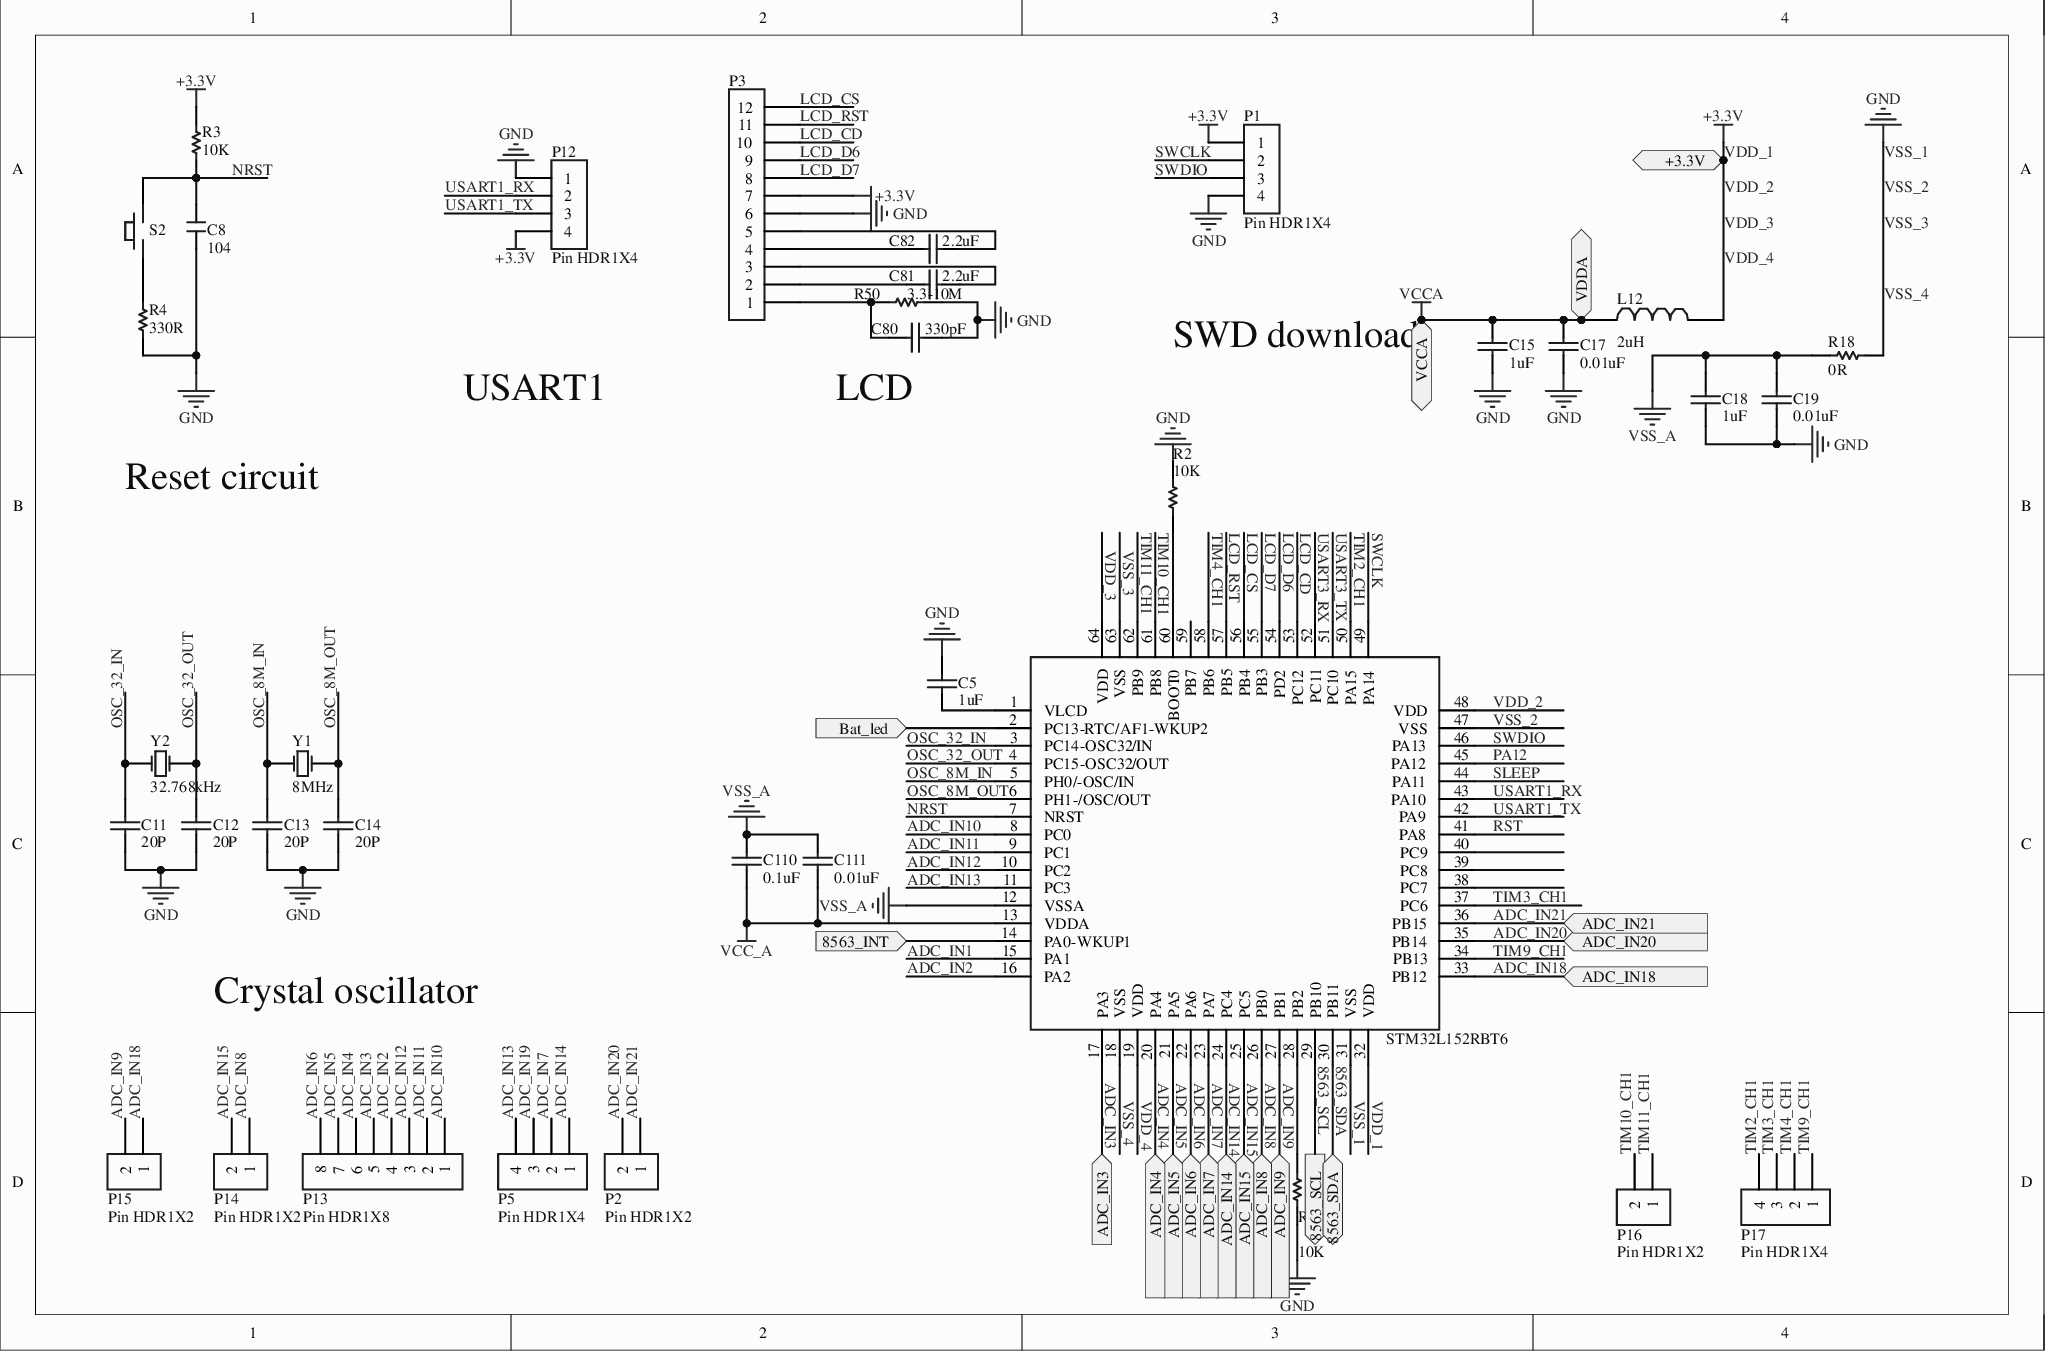
[diagram p0: MISC51920-3.schdoc]
# Altium project MISC51920-2.PrjPcb
1 sheet, 36 parts. Net scope: flat (ports and power ports of the same name join across sheets).
Board file: MISC51920.pcbdoc

## Sheet MISC51920-3.schdoc
size 292 x 193 mm; SheetNumber: 1; SheetTotal: 1; Name: MISC51920

### Parts
C5  1uF  [C 0603]
C8  104  [C 0603]
C11  20P  [C 0603]
C12  20P  [C 0603]
C13  20P  [C 0603]
C14  20P  [C 0603]
C15  1uF  [C 0603]
C17  0.01uF  [C 0603]
C18  1uF  [C 0603]
C19  0.01uF  [C 0603]
C80  330pF  [C 0603]
C81  2.2uF  [C 0603]
C82  2.2uF  [C 0603]
C110  0.1uF  [C 0603]
C111  0.01uF  [C 0603]
L12  2uH  [R 0603]
P1  Pin HDR1X4  [Pin HDR1X4/2.54mm-S]
P2  Pin HDR1X2  [Pin HDR1X2/2.54mm-S]
P3  Pin HDR1X12  [Pin HDR1X12/2.54mm-S]  (value not drawn)
P5  Pin HDR1X4  [Pin HDR1X4/2.54mm-S]
P12  Pin HDR1X4  [Pin HDR1X4/2.54mm-S]
P13  Pin HDR1X8  [Pin HDR1X8/2.54mm-S]
P14  Pin HDR1X2  [Pin HDR1X2/2.54mm-S]
P15  Pin HDR1X2  [Pin HDR1X2/2.54mm-S]
P16  Pin HDR1X2  [Pin HDR1X2/2.54mm-S]
P17  Pin HDR1X4  [Pin HDR1X4/2.54mm-S]
R1  10K  [0603R]
R2  10K  [0603R]
R3  10K  [0603R]
R4  330R  [0603R]
R18  0R  [0603R]
R50  3.3-10M  [0603R]
S2  KEY  [SWTP3.7X6]  (value not drawn)
U1  STM32L152RBT6  [LQFP-64_L10.0-W10.0-P0.50-LS12.0-BL]
Y1  8MHz  [XTAL_SMD49S]
Y2  32.768kHz  [OSC 3215-2P]

### Ports
8563_INT (in), 8563_SCL (out), 8563_SDA (bidir), +3.3V (bidir), ADC_IN3 (in), ADC_IN4 (in), ADC_IN5 (in), ADC_IN6 (in), ADC_IN7 (in), ADC_IN8 (in), ADC_IN9 (in), ADC_IN14 (in), ADC_IN15 (in), ADC_IN18 (in), ADC_IN20 (in), ADC_IN21 (in), Bat_led (in), VCCA (bidir), VDDA (bidir)

### Nets
VCC_A: C110.2 C111.2 U1.13(VDDA)
VCCA: C15.2 C17.2 L12.1 ; port VCCA, port VDDA
+3.3V: L12.2 P1.1 P3.7 P12.4 R3.2 U1.19(VDD) U1.32(VDD) U1.48(VDD) U1.64(VDD) ; port +3.3V  [also labelled VDD_1, VDD_2, VDD_3, VDD_4]
VSS_1: C5.1 C8.1 C11.1 C12.2 C13.1 C14.2 C15.1 C17.1 C18.1 C19.1 C80.2 P1.4 P3.6 P12.1 R1.1 R2.2 R4.1 R18.1 R50.1 U1.18(VSS) U1.31(VSS) U1.47(VSS) U1.63(VSS)  [also labelled GND, VSS_2, VSS_3, VSS_4]
VSS_A: C18.2 C19.2 C110.1 C111.1 R18.2 U1.12(VSSA)
8563_SCL: U1.29(PB10) ; port 8563_SCL
8563_SDA: U1.30(PB11) ; port 8563_SDA
ADC_IN1: U1.15(PA1)
ADC_IN2: P13.4 U1.16(PA2)
ADC_IN3: P13.5 U1.17(PA3) ; port ADC_IN3
ADC_IN4: P13.6 U1.20(PA4) ; port ADC_IN4
ADC_IN5: P13.7 U1.21(PA5) ; port ADC_IN5
ADC_IN6: P13.8 U1.22(PA6) ; port ADC_IN6
ADC_IN7: P5.2 U1.23(PA7) ; port ADC_IN7
ADC_IN8: P14.1 U1.26(PB0) ; port ADC_IN8
ADC_IN9: P15.2 U1.27(PB1) ; port ADC_IN9
ADC_IN10: P13.1 U1.8(PC0)
ADC_IN11: P13.2 U1.9(PC1)
ADC_IN12: P13.3 U1.10(PC2)
ADC_IN13: P5.4 U1.11(PC3)
ADC_IN14: P5.1 U1.24(PC4) ; port ADC_IN14
ADC_IN15: P14.2 U1.25(PC5) ; port ADC_IN15
ADC_IN18: P15.1 U1.33(PB12) ; port ADC_IN18
ADC_IN19: P5.3
ADC_IN20: P2.2 U1.35(PB14) ; port ADC_IN20
ADC_IN21: P2.1 U1.36(PB15) ; port ADC_IN21
LCD_CD: P3.10 U1.53(PC12)
LCD_CS: P3.12 U1.56(PB4)
LCD_D6: P3.9 U1.54(PD2)
LCD_D7: P3.8 U1.55(PB3)
LCD_RST: P3.11 U1.57(PB5)
NRST: C8.2 R3.1 S2.2 U1.7(NRST)
OSC_8M_IN: C13.2 U1.5(PH0/-OSC/IN) Y1.2(OSC2)
OSC_8M_OUT: C14.1 U1.6(PH1-/OSC/OUT) Y1.1(OSC1)
OSC_32_IN: C11.2 U1.3(PC14-OSC32/IN) Y2.1(OSC1)
OSC_32_OUT: C12.1 U1.4(PC15-OSC32/OUT) Y2.2(OSC2)
PA12: U1.45(PA12)
RST: U1.41(PA8)
SLEEP: U1.44(PA11)
SWCLK: P1.2 U1.49(PA14)
SWDIO: P1.3 U1.46(PA13)
TIM2_CH1: P17.4 U1.50(PA15)
TIM3_CH1: P17.3 U1.37(PC6)
TIM4_CH1: P17.2 U1.58(PB6)
TIM9_CH1: P17.1 U1.34(PB13)
TIM10_CH1: P16.2 U1.61(PB8)
TIM11_CH1: P16.1 U1.62(PB9)
USART1_RX: P12.2 U1.43(PA10)
USART1_TX: P12.3 U1.42(PA9)
USART3_RX: U1.52(PC11)
USART3_TX: U1.51(PC10)
NetC5_2: C5.2 U1.1(VLCD)
NetC80_1: C80.1 P3.1 R50.2
NetC81_1: C81.1 P3.2
NetC81_2: C81.2 P3.3
NetC82_1: C82.1 P3.4
NetC82_2: C82.2 P3.5
NetR1_2: R1.2 U1.28(PB2)
NetR2_1: R2.1 U1.60(BOOT0)
NetR4_2: R4.2 S2.1
NetU1_2: U1.2(PC13-RTC/AF1-WKUP2) ; port Bat_led
NetU1_14: U1.14(PA0-WKUP1) ; port 8563_INT

Not connected (* = marked no-connect by the designer): U1 38(PC7) 39(PC8) 40(PC9) 59(PB7)

### Notes on the sheet
- USART1
- (near C80) LCD
- SWD download
- Reset circuit
- Crystal oscillator

### Library data of the parts
C5 = C_1: Capacitor; Origin Footprint: C0603; OriginFootprint 2: C0805; OriginFootprint 3: C 0805; UniqueId: ddba3c46cf8b8e66; SymbolName: C; AddInBom: yes; Device: C_1; Published: 8-Jun-2000; LatestRevisionDate: 17-Jul-2002; LatestRevisionNote: Re-released for DXP Platform.; PackageReference: RAD-0.3; PackageDescription: Radial Cap, Thru-Hole; 2 Leads; 0.3 in Pin Spacing; DesignItemID: C; LibraryName: Devices; FootprintName: C 0603; Publisher: Altium Limited
C8 = C: Non-polar chip capacitor; 版权归属: COMPANY_A; Origin Footprint: C 0201; OriginFootprint 2: C 0402; OriginFootprint 3: C 0805; OriginFootprint 4: C 1206; OriginFootprint 5: C 1210; OriginFootprint 6: C 1808; OriginFootprint 7: C 1812; OriginFootprint 8: C 1825; OriginFootprint 9: C 2225; UniqueId: 80f3708378e3d903; AddInBom: yes; Device: C; BOM名称: Non-polar chip capacitor; DesignItemID: C; LibraryName: Resistor-Capacitor-Inductor; SymbolName: C; FootprintName: C 0603
C11 = C_2: Capacitor; Origin Footprint: C0603; OriginFootprint 2: C0805; OriginFootprint 3: C 0805; UniqueId: 20764de07767b3a1; SymbolName: C; AddInBom: yes; Device: C_2; Published: 8-Jun-2000; LatestRevisionDate: 17-Jul-2002; LatestRevisionNote: Re-released for DXP Platform.; PackageReference: RAD-0.3; PackageDescription: Radial Cap, Thru-Hole; 2 Leads; 0.3 in Pin Spacing; DesignItemID: C; LibraryName: Devices; FootprintName: C 0603; Publisher: Altium Limited
C12 = C_1: Capacitor; Origin Footprint: C0603; OriginFootprint 2: C0805; OriginFootprint 3: C 0805; UniqueId: 26a39bcafcc8ce7c; SymbolName: C; AddInBom: yes; Device: C_1; Published: 8-Jun-2000; LatestRevisionDate: 17-Jul-2002; LatestRevisionNote: Re-released for DXP Platform.; PackageReference: RAD-0.3; PackageDescription: Radial Cap, Thru-Hole; 2 Leads; 0.3 in Pin Spacing; DesignItemID: C; LibraryName: Devices; FootprintName: C 0603; Publisher: Altium Limited
C13 = C_1: Capacitor; Origin Footprint: C0603; OriginFootprint 2: C0805; OriginFootprint 3: C 0805; UniqueId: e7ba3aba9f9889c8; SymbolName: C; AddInBom: yes; Device: C_1; Published: 8-Jun-2000; LatestRevisionDate: 17-Jul-2002; LatestRevisionNote: Re-released for DXP Platform.; PackageReference: RAD-0.3; PackageDescription: Radial Cap, Thru-Hole; 2 Leads; 0.3 in Pin Spacing; DesignItemID: C; LibraryName: Devices; FootprintName: C 0603; Publisher: Altium Limited
C14 = C_1: Capacitor; Origin Footprint: C0603; OriginFootprint 2: C0805; OriginFootprint 3: C 0805; UniqueId: 00361082df9d4549; SymbolName: C; AddInBom: yes; Device: C_1; Published: 8-Jun-2000; LatestRevisionDate: 17-Jul-2002; LatestRevisionNote: Re-released for DXP Platform.; PackageReference: RAD-0.3; PackageDescription: Radial Cap, Thru-Hole; 2 Leads; 0.3 in Pin Spacing; DesignItemID: C; LibraryName: Devices; FootprintName: C 0603; Publisher: Altium Limited
C15 = C_1: Capacitor; Origin Footprint: C0603; OriginFootprint 2: C0805; OriginFootprint 3: C 0805; UniqueId: 86bb77bda672094d; SymbolName: C; AddInBom: yes; Device: C_1; Published: 8-Jun-2000; LatestRevisionDate: 17-Jul-2002; LatestRevisionNote: Re-released for DXP Platform.; PackageReference: RAD-0.3; PackageDescription: Radial Cap, Thru-Hole; 2 Leads; 0.3 in Pin Spacing; DesignItemID: C; LibraryName: Devices; FootprintName: C 0603; Publisher: Altium Limited
C17 = C_1: Capacitor; Origin Footprint: C0603; OriginFootprint 2: C0805; OriginFootprint 3: C 0805; UniqueId: 48700c84863a802e; SymbolName: C; AddInBom: yes; Device: C_1; Published: 8-Jun-2000; LatestRevisionDate: 17-Jul-2002; LatestRevisionNote: Re-released for DXP Platform.; PackageReference: RAD-0.3; PackageDescription: Radial Cap, Thru-Hole; 2 Leads; 0.3 in Pin Spacing; DesignItemID: C; LibraryName: Devices; FootprintName: C 0603; Publisher: Altium Limited
C18 = C_1: Capacitor; Origin Footprint: C0603; OriginFootprint 2: C0805; OriginFootprint 3: C 0805; UniqueId: d9d0285421fe3ef0; SymbolName: C; AddInBom: yes; Device: C_1; Published: 8-Jun-2000; LatestRevisionDate: 17-Jul-2002; LatestRevisionNote: Re-released for DXP Platform.; PackageReference: RAD-0.3; PackageDescription: Radial Cap, Thru-Hole; 2 Leads; 0.3 in Pin Spacing; DesignItemID: C; LibraryName: Devices; FootprintName: C 0603; Publisher: Altium Limited
C19 = C_1: Capacitor; Origin Footprint: C0603; OriginFootprint 2: C0805; OriginFootprint 3: C 0805; UniqueId: 9b75bd895f0e39d2; SymbolName: C; AddInBom: yes; Device: C_1; Published: 8-Jun-2000; LatestRevisionDate: 17-Jul-2002; LatestRevisionNote: Re-released for DXP Platform.; PackageReference: RAD-0.3; PackageDescription: Radial Cap, Thru-Hole; 2 Leads; 0.3 in Pin Spacing; DesignItemID: C; LibraryName: Devices; FootprintName: C 0603; Publisher: Altium Limited
C80 = C_1: Capacitor; Origin Footprint: C0603; OriginFootprint 2: C0805; OriginFootprint 3: C 0805; UniqueId: 2dbd9816442fdb9a; SymbolName: C; AddInBom: yes; Device: C_1; Published: 8-Jun-2000; LatestRevisionDate: 17-Jul-2002; LatestRevisionNote: Re-released for DXP Platform.; PackageReference: RAD-0.3; PackageDescription: Radial Cap, Thru-Hole; 2 Leads; 0.3 in Pin Spacing; DesignItemID: C; LibraryName: Devices; FootprintName: C 0603; Publisher: Altium Limited
C81 = C_1: Capacitor; Origin Footprint: C0603; OriginFootprint 2: C0805; OriginFootprint 3: C 0805; UniqueId: bdf2686215596067; SymbolName: C; AddInBom: yes; Device: C_1; Published: 8-Jun-2000; LatestRevisionDate: 17-Jul-2002; LatestRevisionNote: Re-released for DXP Platform.; PackageReference: RAD-0.3; PackageDescription: Radial Cap, Thru-Hole; 2 Leads; 0.3 in Pin Spacing; DesignItemID: C; LibraryName: Devices; FootprintName: C 0603; Publisher: Altium Limited
C82 = C_1: Capacitor; Origin Footprint: C0603; OriginFootprint 2: C0805; OriginFootprint 3: C 0805; UniqueId: 2ac4a713bdb27458; SymbolName: C; AddInBom: yes; Device: C_1; Published: 8-Jun-2000; LatestRevisionDate: 17-Jul-2002; LatestRevisionNote: Re-released for DXP Platform.; PackageReference: RAD-0.3; PackageDescription: Radial Cap, Thru-Hole; 2 Leads; 0.3 in Pin Spacing; DesignItemID: C; LibraryName: Devices; FootprintName: C 0603; Publisher: Altium Limited
C110 = C_1: Capacitor; Origin Footprint: C0603; OriginFootprint 2: C0805; OriginFootprint 3: C 0805; UniqueId: 650bdd21373e6b88; SymbolName: C; AddInBom: yes; Device: C_1; Published: 8-Jun-2000; LatestRevisionDate: 17-Jul-2002; LatestRevisionNote: Re-released for DXP Platform.; PackageReference: RAD-0.3; PackageDescription: Radial Cap, Thru-Hole; 2 Leads; 0.3 in Pin Spacing; DesignItemID: C; LibraryName: Devices; FootprintName: C 0603; Publisher: Altium Limited
C111 = C_3: Capacitor; Origin Footprint: C0603; OriginFootprint 2: C0805; OriginFootprint 3: C 0805; UniqueId: c0e8232d23165c04; SymbolName: C; AddInBom: yes; Device: C_3; Published: 8-Jun-2000; LatestRevisionDate: 17-Jul-2002; LatestRevisionNote: Re-released for DXP Platform.; PackageReference: RAD-0.3; PackageDescription: Radial Cap, Thru-Hole; 2 Leads; 0.3 in Pin Spacing; DesignItemID: C; LibraryName: Devices; FootprintName: C 0603; Publisher: Altium Limited
L12 = INDUCTOR: Origin Footprint: AL0204; OriginFootprint 2: AL0204_V; OriginFootprint 3: AL0307; OriginFootprint 4: AL0307_V; OriginFootprint 5: AL0410; OriginFootprint 6: AL0410_V; OriginFootprint 7: AL0510; OriginFootprint 8: AL0510_V; OriginFootprint 9: CD31; OriginFootprint 10: CD32; OriginFootprint 11: CD42; OriginFootprint 12: CD43; OriginFootprint 13: CD52; OriginFootprint 14: CD53; OriginFootprint 15: CD54; OriginFootprint 16: CD75; OriginFootprint 17: CD104; OriginFootprint 18: CD105; OriginFootprint 19: CD106; OriginFootprint 20: CDRH73; OriginFootprint 21: CDRH74; OriginFootprint 22: CDRH124; OriginFootprint 23: CDRH125; OriginFootprint 24: CDRH127; OriginFootprint 25: CDRH129; OriginFootprint 26: L 0630; OriginFootprint 27: NR3015; OriginFootprint 28: PK0406; OriginFootprint 29: PK0608; OriginFootprint 30: PK0810; OriginFootprint 31: PK0912; OriginFootprint 32: PK1012; OriginFootprint 33: PK1415; OriginFootprint 34: PK1618; OriginFootprint 35: PK1818; OriginFootprint 36: 0402L; OriginFootprint 37: 0603L; OriginFootprint 38: 0630L; OriginFootprint 39: 0805L; OriginFootprint 40: 1210L; OriginFootprint 41: Model Name; OriginFootprint 42: 1806L; OriginFootprint 43: 1812L; UniqueId: 17da6896838d082f; AddInBom: yes; Device: INDUCTOR; OriginFootprint 44: R 0603; DesignItemID: INDUCTOR; LibraryName: Inductor; Description: INDUCTOR; SymbolName: INDUCTOR; FootprintName: R 0603
P1 = Pin HDR1X4_1: Origin Footprint: Pin HDR1X4/2.54mm-W; UniqueId: c39ee3c861a7b382; AddInBom: yes; Device: Pin HDR1X4_1; DesignItemID: Pin HDR1X4; LibraryName: Pin header; SymbolName: Pin HDR1X4; FootprintName: Pin HDR1X4/2.54mm-S
P2 = Pin HDR1X2: Origin Footprint: Pin HDR1X2/2.54mm-W; UniqueId: 16cbebb8866e1842; AddInBom: yes; Device: Pin HDR1X2; DesignItemID: Pin HDR1X2; LibraryName: Pin header; SymbolName: Pin HDR1X2; FootprintName: Pin HDR1X2/2.54mm-S
P3 = Pin HDR1X12: OriginFootprint 2: Pin HDR1X12/2.54mm-W; OriginFootprint 3: LCD-TH_HS12864G06BN; UniqueId: 1bc31e334497ec54; AddInBom: yes; Device: Pin HDR1X12; Origin Footprint: Pin HDR1X12/2.54mm-S; DesignItemID: Pin HDR1X12; LibraryName: Pin header; SymbolName: Pin HDR1X12; FootprintName: Pin HDR1X12/2.54mm-S
P5 = Pin HDR1X4: Origin Footprint: Pin HDR1X4/2.54mm-W; UniqueId: a30bd92ff87464e3; AddInBom: yes; Device: Pin HDR1X4; DesignItemID: Pin HDR1X4; LibraryName: Pin header; SymbolName: Pin HDR1X4; FootprintName: Pin HDR1X4/2.54mm-S
P12 = Pin HDR1X4_1: Origin Footprint: Pin HDR1X4/2.54mm-W; UniqueId: 0618e235635c86ae; AddInBom: yes; Device: Pin HDR1X4_1; DesignItemID: Pin HDR1X4; LibraryName: Pin header; SymbolName: Pin HDR1X4; FootprintName: Pin HDR1X4/2.54mm-S
P13 = Pin HDR1X8: Origin Footprint: Pin HDR1X8/2.54mm-W; UniqueId: 57faa0d66134c9f8; AddInBom: yes; Device: Pin HDR1X8; DesignItemID: Pin HDR1X8; LibraryName: Pin header; SymbolName: Pin HDR1X8; FootprintName: Pin HDR1X8/2.54mm-S
P14 = Pin HDR1X2: Origin Footprint: Pin HDR1X2/2.54mm-W; UniqueId: a82060a4d9aa0a79; AddInBom: yes; Device: Pin HDR1X2; DesignItemID: Pin HDR1X2; LibraryName: Pin header; SymbolName: Pin HDR1X2; FootprintName: Pin HDR1X2/2.54mm-S
P15 = Pin HDR1X2: Origin Footprint: Pin HDR1X2/2.54mm-W; UniqueId: c9f4540a6f6f83ef; AddInBom: yes; Device: Pin HDR1X2; DesignItemID: Pin HDR1X2; LibraryName: Pin header; SymbolName: Pin HDR1X2; FootprintName: Pin HDR1X2/2.54mm-S
P16 = Pin HDR1X2: Origin Footprint: Pin HDR1X2/2.54mm-W; UniqueId: 85de28bb97675377; AddInBom: yes; Device: Pin HDR1X2; DesignItemID: Pin HDR1X2; LibraryName: Pin header; SymbolName: Pin HDR1X2; FootprintName: Pin HDR1X2/2.54mm-S
P17 = Pin HDR1X4: Origin Footprint: Pin HDR1X4/2.54mm-W; UniqueId: 4590d5dc20d79a81; AddInBom: yes; Device: Pin HDR1X4; DesignItemID: Pin HDR1X4; LibraryName: Pin header; SymbolName: Pin HDR1X4; FootprintName: Pin HDR1X4/2.54mm-S
R1 = RES0603: Resistor; Origin Footprint: R0603; OriginFootprint 2: R 0805; UniqueId: 353b166cc2dee846; AddInBom: yes; Device: RES0603; Published: 8-Jun-2000; LatestRevisionDate: 17-Jul-2002; LatestRevisionNote: Re-released for DXP Platform.; PackageReference: AXIAL-0.3; PackageDescription: Axial Device, Thru-Hole; 2 Leads; 0.3 in Pin Spacing; DesignItemID: RES0603; LibraryName: Devices; SymbolName: RES0603; FootprintName: 0603R; Publisher: Altium Limited
R2 = RES0603: Resistor; Origin Footprint: R0603; OriginFootprint 2: R 0805; UniqueId: 6f63fc6711cfa315; AddInBom: yes; Device: RES0603; Published: 8-Jun-2000; LatestRevisionDate: 17-Jul-2002; LatestRevisionNote: Re-released for DXP Platform.; PackageReference: AXIAL-0.3; PackageDescription: Axial Device, Thru-Hole; 2 Leads; 0.3 in Pin Spacing; DesignItemID: RES0603; LibraryName: Devices; SymbolName: RES0603; FootprintName: 0603R; Publisher: Altium Limited
R3 = RES0603: Resistor; Origin Footprint: R0603; OriginFootprint 2: R 0805; UniqueId: fe89d0632cfce75f; AddInBom: yes; Device: RES0603; Published: 8-Jun-2000; LatestRevisionDate: 17-Jul-2002; LatestRevisionNote: Re-released for DXP Platform.; PackageReference: AXIAL-0.3; PackageDescription: Axial Device, Thru-Hole; 2 Leads; 0.3 in Pin Spacing; DesignItemID: RES0603; LibraryName: Devices; SymbolName: RES0603; FootprintName: 0603R; Publisher: Altium Limited
R4 = RES0603_1: Resistor; Origin Footprint: R0603; OriginFootprint 2: R 0805; UniqueId: fdc86a4b576d9e98; AddInBom: yes; Device: RES0603_1; Published: 8-Jun-2000; LatestRevisionDate: 17-Jul-2002; LatestRevisionNote: Re-released for DXP Platform.; PackageReference: AXIAL-0.3; PackageDescription: Axial Device, Thru-Hole; 2 Leads; 0.3 in Pin Spacing; DesignItemID: RES0603; LibraryName: Devices; SymbolName: RES0603; FootprintName: 0603R; Publisher: Altium Limited
R18 = RES0603: Resistor; Origin Footprint: R0603; OriginFootprint 2: R 0805; UniqueId: 5f673669f0d56d8f; AddInBom: yes; Device: RES0603; Published: 8-Jun-2000; LatestRevisionDate: 17-Jul-2002; LatestRevisionNote: Re-released for DXP Platform.; PackageReference: AXIAL-0.3; PackageDescription: Axial Device, Thru-Hole; 2 Leads; 0.3 in Pin Spacing; DesignItemID: RES0603; LibraryName: Devices; SymbolName: RES0603; FootprintName: 0603R; Publisher: Altium Limited
R50 = RES0603_2: Resistor; Origin Footprint: R0603; OriginFootprint 2: R 0805; UniqueId: a074999702fa02e6; AddInBom: yes; Device: RES0603_2; Published: 8-Jun-2000; LatestRevisionDate: 17-Jul-2002; LatestRevisionNote: Re-released for DXP Platform.; PackageReference: AXIAL-0.3; PackageDescription: Axial Device, Thru-Hole; 2 Leads; 0.3 in Pin Spacing; DesignItemID: RES0603; LibraryName: Devices; SymbolName: RES0603; FootprintName: 0603R; Publisher: Altium Limited
S2 = KEY: Ordinary tactile button; Origin Footprint: KEY-12X12X7.5; OriginFootprint 2: DSW-KEY-SOT-4_5x4_5; OriginFootprint 3: DSW-KFC-022S-H2.5; OriginFootprint 4: TSW DIP-6*6*4.3; OriginFootprint 5: TSW SMD-3*6*5; UniqueId: 16ca49f37df57620; AddInBom: yes; Device: KEY; DesignItemID: KEY; LibraryName: Devices; SymbolName: KEY; FootprintName: SWTP3.7X6
U1 = STM32L152RBT6: UniqueId: 1bdc0ab44f99f92d; AddInBom: yes; Device: STM32L152RBT6; DesignItemID: STM32L152RBT6; LibraryName: GC3M0015065KGC3M0015065K; SymbolName: STM32L152RBT6; FootprintName: LQFP-64_L10.0-W10.0-P0.50-LS12.0-BL
Y1 = XTAL: Crystal Oscillator; Origin Footprint: X-DT-26; OriginFootprint 2: X-HC49-SMT; OriginFootprint 3: X-HC49S; OriginFootprint 4: X-MC146; OriginFootprint 5: X-NX5032GA; OriginFootprint 6: XTAL-49S DIP; UniqueId: 9790cc8ece124e27; AddInBom: yes; Device: XTAL; Published: 8-Jun-2000; LatestRevisionDate: 17-Jul-2002; LatestRevisionNote: Re-released for DXP Platform.; DesignItemID: XTAL; LibraryName: Devices; SymbolName: XTAL; FootprintName: XTAL_SMD49S; Publisher: Altium Limited
Y2 = XTAL_1: Crystal Oscillator; Origin Footprint: X-DT-26; OriginFootprint 2: X-HC49-SMT; OriginFootprint 3: X-HC49S; OriginFootprint 4: X-MC146; OriginFootprint 5: X-NX5032GA; OriginFootprint 6: MC-146_4P-L6.7-W1.5-P0.85-TL; UniqueId: 54aa28710a128dff; SymbolName: XTAL; AddInBom: yes; Device: XTAL_1; Published: 8-Jun-2000; LatestRevisionDate: 17-Jul-2002; LatestRevisionNote: Re-released for DXP Platform.; OriginFootprint 7: XTAL-3215; DesignItemID: XTAL; LibraryName: Devices; FootprintName: OSC 3215-2P; Publisher: Altium Limited